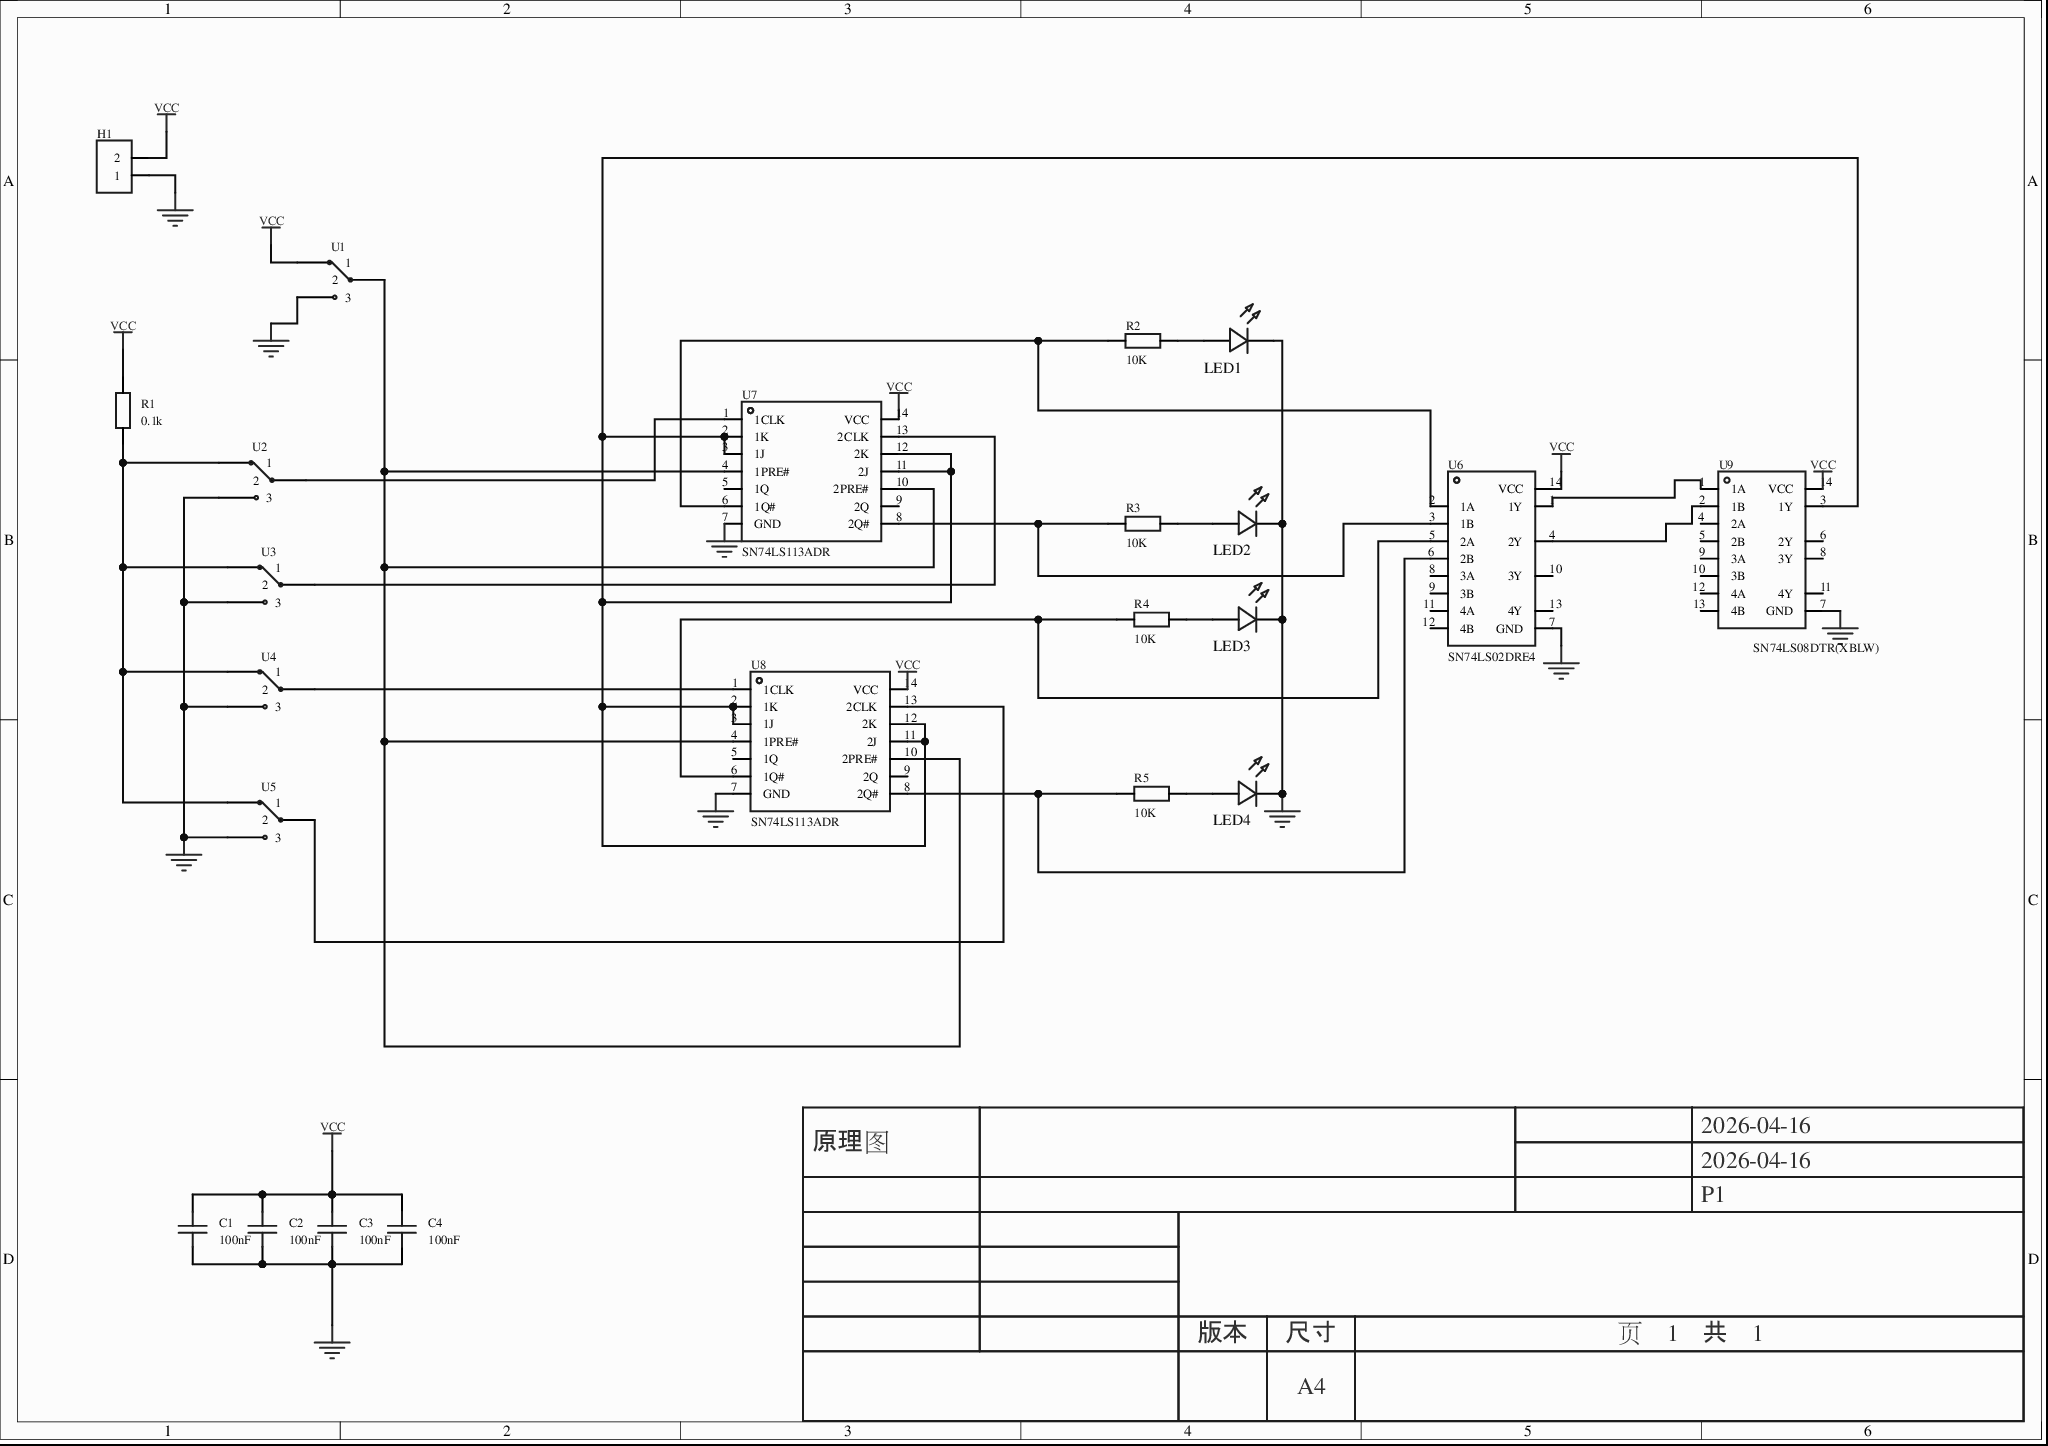
[diagram p0: MISC51255-3.schdoc]
# Altium project MISC51255-2.PrjPcb
1 sheet, 23 parts. Net scope: global (net labels, ports and power ports of the same name join across sheets).
Board file: MISC51255.pcbdoc

## Sheet MISC51255-3.schdoc
size 297 x 209 mm; Version: V1.0; @Project Name: MISC51255; @Page Count: 1; @Update Date: 2026-04-19; @Create Date: 2026-04-19; @Schematic Name: MISC51255; @Page No: 1; @Create Time: 08:37:13; @Update Time: 08:37:13; @Board Name: MISC51255

### Parts
C1  100nF  [C0603]
C2  100nF  [C0603]
C3  100nF  [C0603]
C4  100nF  [C0603]
H1  (no value)  [HDR-TH_2P-P2.54-V-F]
LED1  (no value)  [LED_0603]
LED2  (no value)  [LED_0603]
LED3  (no value)  [LED_0603]
LED4  (no value)  [LED_0603]
R1  0.1k  [R0603]
R2  10K  [R0603]
R3  10K  [R0603]
R4  10K  [R0603]
R5  10K  [R0603]
U1  (no value)  [单刀双掷]
U2  (no value)  [单刀双掷]
U3  (no value)  [单刀双掷]
U4  (no value)  [单刀双掷]
U5  (no value)  [单刀双掷]
U6  SN74LS02DRE4  [SOIC-14_L8.7-W3.9-P1.27-LS6.0-BL]
U7  SN74LS113ADR  [SOIC-14_L8.6-W3.9-P1.27-LS6.0-BL]
U8  SN74LS113ADR  [SOIC-14_L8.6-W3.9-P1.27-LS6.0-BL]
U9  SN74LS08DTR(XBLW)  [SOIC-14_L8.7-W3.9-P1.27-LS6.0-BL]

### Nets
GND: C1.1 C2.1 C3.1 C4.1 H1.1 LED1.1(C) LED2.1(C) LED3.1(C) LED4.1(C) U1.3 U2.3 U3.3 U4.3 U5.3 U6.7(GND) U7.7(GND) U8.7(GND) U9.7(GND)
VCC: C1.2 C2.2 C3.2 C4.2 H1.2 R1.2 U1.1 U6.14(VCC) U7.14(VCC) U8.14(VCC) U9.14(VCC)
NetLED1_2: LED1.2(A) R2.2
NetLED2_2: LED2.2(A) R3.2
NetLED3_2: LED3.2(A) R4.2
NetLED4_2: LED4.2(A) R5.2
NetR1_1: R1.1 U2.1 U3.1 U4.1 U5.1
NetR2_1: R2.1 U6.2(1A) U7.6(1Q#)
NetR3_1: R3.1 U6.3(1B) U7.8(2Q#)
NetR4_1: R4.1 U6.5(2A) U8.6(1Q#)
NetR5_1: R5.1 U6.6(2B) U8.8(2Q#)
NetU1_2: U1.2 U7.4(1PRE#) U7.10(2PRE#) U8.4(1PRE#) U8.10(2PRE#)
NetU2_2: U2.2 U7.1(1CLK)
NetU3_2: U3.2 U7.13(2CLK)
NetU4_2: U4.2 U8.1(1CLK)
NetU5_2: U5.2 U8.13(2CLK)
NetU6_1: U6.1(1Y) U9.1(1A)
NetU6_4: U6.4(2Y) U9.2(1B)
NetU7_2: U7.2(1K) U7.3(1J) U7.11(2J) U7.12(2K) U8.2(1K) U8.3(1J) U8.11(2J) U8.12(2K) U9.3(1Y)

Not connected (* = marked no-connect by the designer): U6 8(3A)* 9(3B)* 10(3Y)* 11(4A)* 12(4B)* 13(4Y)*; U7 5(1Q)* 9(2Q)*; U8 5(1Q)* 9(2Q)*; U9 4(2A)* 5(2B)* 6(2Y)* 8(3Y)* 9(3A)* 10(3B)* 11(4Y)* 12(4A)* 13(4B)*

### Notes on the sheet
- 2026-04-16
- 原理图
- P1
- 版本
- 尺寸
- A4
- 页    1    共    1

### Library data of the parts
C1-C4 = CAP_0603: Symbol: CapAcitance; ConvertToPcb: yes; ModelId: ac125912035d415993ca9572d50418b10819f05c4eef4c71ace90d822a990e87; ModelName: C0603_L1.6-W0.8-H0.8; ModelTransform: 62.992,31.496,0,0,0,0,0,0,0; Device: CAP_0603; FootprintName: C0603; AddInBom: yes; Supplier Footprint: 0603; Value: 100nF
H1 = HDR-F_2.54_1x2P: Manufacturer: BOOMELE(博穆精密); Manufacturer Part: 2.54-1*2P母; Symbol: Header-Female-2.54_1x2; ConvertToPcb: yes; ModelId: a9450ef445564560a104363b9aacde4e0819f05c4eef4c71ace90d822a990e87; ModelName: HDR-TH_2P-P2.54-F-LI-1X2P; ModelTransform: 215.7476,98.425,0,0,0,0,0,0,-129.921; Device: HDR-F_2.54_1x2P; Supplier: LCSC; Supplier Part: C49661; JLCPCB Part Class: Extended Part; FootprintName: HDR-TH_2P-P2.54-V-F; AddInBom: yes; Supplier Footprint: 插件
LED1-LED4 = LED_0603-R: Symbol: LED_R; Convert to PCB: yes; 3D Model: dd8257b0d61a4cd7b68939a056e080950819f05c4eef4c71ace90d822a990e87; 3D Model Transform: 58.72,29.4,22.03,0,0,0,0,0,0; ModelName: LED-0603_R; Device: LED_0603-R; Add into BOM: yes; Supplier Footprint: 0603; FootprintName: LED_0603
R1-R5 = Res_0603: Symbol: 电阻; ConvertToPcb: yes; ModelId: fc143cca1e79419f9cd78b61e9279f080819f05c4eef4c71ace90d822a990e87; ModelTransform: 31.8897,63.7794,0,90,0,0,0,0,0; Device: Res_0603; FootprintName: R0603; AddInBom: yes; Supplier Footprint: 0603; ModelName: R0603
  R1: Value: 0.1k
  R2-R5: Value: 10K
U1-U5 = 单刀双掷开关: AddInBom: yes; Device: 单刀双掷开关; Symbol: 单刀双掷开关; FootprintName: 单刀双掷; ConvertToPcb: yes
U6 = SN74LS02DRE4: 逻辑类型:或非门;通道数:4;工作电压:4.75V~5.25V;传播延迟(tpd):15ns@5V,15pF;; Manufacturer: TI(德州仪器); AddInBom: yes; Logic Type: 或非门; Number of Channels: 4; Current - Output Low(IOL): 8mA; Current - Output High(IOH): 400uA; Input Logic Level - High: 2V; Input Logic Level - Low: 800mV; Output Logic Level - High: 2.7V; Output Logic Level - Low: 500mV; Input Number: 2; ModelId: 8dbf5b715d42428c85558507ae5a252b0819f05c4eef4c71ace90d822a990e87; ModelName: SOIC-14_L8.6-W3.9-H1.8-LS6.0-P1.27; ModelTransform: 338.583,236.22,0,0,0,0,0,0.001,0; Device: SN74LS02DRE4; Symbol: SN74LS02DRE4; FootprintName: SOIC-14_L8.7-W3.9-P1.27-LS6.0-BL; LCSC Part Name: SN74LS02DRE4; SupplierPart: C4472094; ManufacturerPart: SN74LS02DRE4; Supplier Footprint: SOIC-14; JLCPCB Part Class: Extended Part; Datasheet: https://www.ti.com/cn/lit/gpn/sn74ls02; Supplier: LCSC; ConvertToPcb: yes; Voltage - Supply: 4.75V~5.25V; Series: 74LS; Propagation Delay: 15ns@5V,15pF; Operating Temperature: 0℃~+70℃
U7 U8 = SN74LS113ADR: Manufacturer: TI(德州仪器); AddInBom: yes; ModelId: 695b8c4936c24917a6b704d8b60c2d4d0819f05c4eef4c71ace90d822a990e87; ModelTransform: 340.5505,236.22,0,0,0,0,0,0,0; Device: SN74LS113ADR; Symbol: SN74LS113ADR; FootprintName: SOIC-14_L8.6-W3.9-P1.27-LS6.0-BL; LCSC Part Name: SN74LS113ADR; SupplierPart: C5755807; ManufacturerPart: SN74LS113ADR; Supplier Footprint: -; JLCPCB Part Class: Extended Part; Datasheet: https://atta.szlcsc.com/upload/public/pdf/source/20230922/26AB19584FB82236BDA08EB995C200CE.pdf; Supplier: LCSC; ConvertToPcb: yes; ModelName: SOIC-14_L8.6-W3.9-P1.27-LS6.0-BL
U9 = SN74LS08DTR(XBLW): Manufacturer: XBLW(芯伯乐); AddInBom: yes; ModelId: 8dbf5b715d42428c85558507ae5a252b0819f05c4eef4c71ace90d822a990e87; ModelName: SOIC-14_L8.6-W3.9-H1.8-LS6.0-P1.27; ModelTransform: 338.583,236.22,0,0,0,0,0,0.001,0; Device: SN74LS08DTR(XBLW); Symbol: SN74LS08DTR(XBLW); FootprintName: SOIC-14_L8.7-W3.9-P1.27-LS6.0-BL; LCSC Part Name: SN74LS08DTR(XBLW); SupplierPart: C54525284; ManufacturerPart: SN74LS08DTR(XBLW); Supplier Footprint: SOP-14; JLCPCB Part Class: Extended Part; Datasheet: https://item.szlcsc.com/datasheet/SN74LS08DTR(XBLW)/57873527.html; Supplier: LCSC; ConvertToPcb: yes